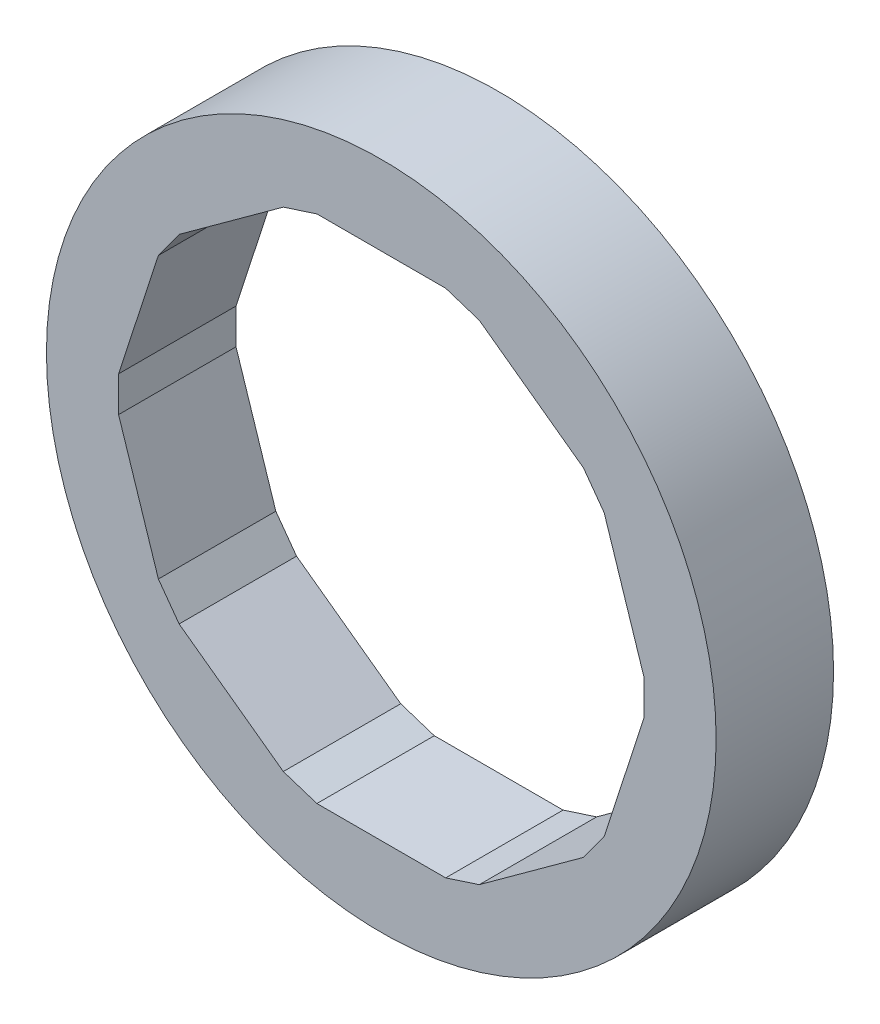
from build123d import *

# Parameters (mm, degrees)
SKETCH_1_R      = 442
EXTRUDE_1_DEPTH = 77.5


with BuildPart() as part:
    # 草图1 → 凸台-拉伸1 (new, symmetric)
    with BuildSketch(Plane.XY):
        Circle(SKETCH_1_R)
        Polygon((346.772490513, -23.298923219), (346.772490513, 23.298923219), (294.23960147, 184.978530989), (266.850074544, 222.676980659), (129.317185501, 322.600473549), (85, 337), (-85, 337), (-129.317185501, 322.600473549), (-266.850074544, 222.676980659), (-294.23960147, 184.978530989), (-346.772490513, 23.298923219), (-346.772490513, -23.298923219), (-294.23960147, -184.978530989), (-266.850074544, -222.676980659), (-129.317185501, -322.600473549), (-85, -337), (85, -337), (129.317185501, -322.600473549), (266.850074544, -222.67698066), (294.23960147, -184.978530989), align=None, mode=Mode.SUBTRACT)
    extrude(amount=EXTRUDE_1_DEPTH, both=True)


solid = part.part
